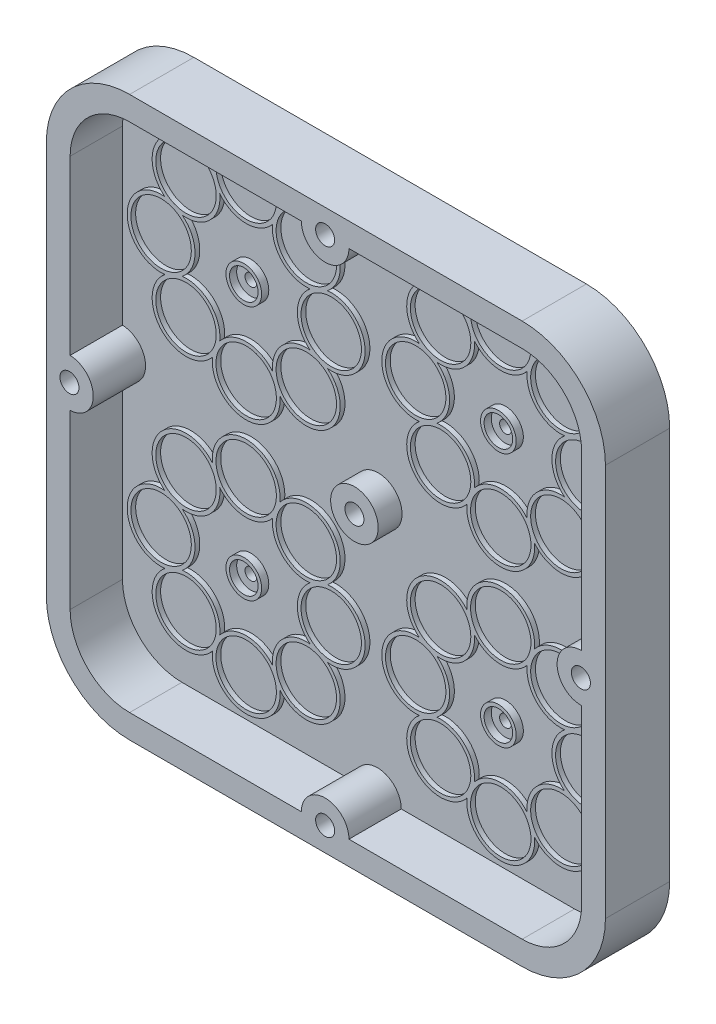
SolidWorks part; units mm, degrees
ref_plane "Front Plane" through (0, 0, 0) normal (0, 0, 1) x (1, 0, 0)
ref_plane "Top Plane" through (0, 0, 0) normal (0, 1, 0) x (1, 0, 0)
ref_plane "Right Plane" through (0, 0, 0) normal (1, 0, 0) x (0, 0, -1)
other "Configuration Table"
sketch "Sketch1" plane through (0, 0, 0) normal (0, 0, 1) x (1, 0, 0)
  line L0 (117.5, 235) -> (117.5, 0) construction
  line L1 (35, 0) -> (200, 0)
  line L2 (0, 35) -> (0, 200)
  line L3 (35, 235) -> (200, 235)
  line L4 (235, 35) -> (235, 200)
  line L5 (0, 117.5) -> (235, 117.5) construction
  line L7 (64, 64) -> (171, 64) construction
  line L8 (64, 64) -> (64, 171) construction
  line L9 (64, 171) -> (171, 171) construction
  line L10 (171, 64) -> (171, 171) construction
  line L11 (64, 64) -> (171, 171) construction
  line L12 (64, 171) -> (171, 64) construction
  arc A0 (200, 0) -> (235, 35) centre (200, 35) ccw
  arc A1 (200, 235) -> (235, 200) centre (200, 200) cw
  arc A2 (35, 0) -> (0, 35) centre (35, 35) cw
  arc A3 (0, 200) -> (35, 235) centre (35, 200) cw
  circle A4 centre (117.5, 225) radius 4
  circle A5 centre (117.5, 10) radius 4
  circle A6 centre (117.5, 117.5) radius 4
  circle A7 centre (225, 117.5) radius 4
  circle A8 centre (10, 117.5) radius 4
  circle A9 centre (64, 171) radius 2.5
  circle A10 centre (171, 171) radius 2.5
  circle A11 centre (171, 64) radius 2.5
  circle A12 centre (64, 64) radius 2.5
  point P7 (235, 0)
  point P12 (0, 0)
  point P15 (0, 235)
  dimension "D3" = 35
  dimension "D4" = 8
  dimension "D5" = 10
  dimension "D6" = 10
  dimension "D7" = 10
  dimension "D8" = 10
  dimension "D11" = 5
  dimension "D1" = 235
  dimension "D2" = 235
  dimension "D9" = 107
  dimension "D10" = 107
extrude "Boss-Extrude1" add sketch "Sketch1" along normal blind 5
sketch "Sketch2" plane through (0, 0, 5) normal (0, 0, 1) x (1, 0, 0)
  line L0 (200, 225) -> (127.186, 225)
  line L1 (10, 200) -> (10, 127.5027)
  line L2 (35, 10) -> (107.186, 10)
  line L3 (225, 35) -> (225, 107.5123)
  line L4 (235, 35) -> (235, 200)
  line L5 (200, 235) -> (35, 235)
  line L6 (0, 200) -> (0, 35)
  line L7 (35, 0) -> (200, 0)
  line L8 (235, 35) -> (235, 200)
  line L9 (200, 235) -> (35, 235)
  line L10 (0, 200) -> (0, 35)
  line L11 (35, 0) -> (200, 0)
  line L12 (10, 107.5104) -> (10, 35)
  line L13 (10, 200) -> (10, 35) construction
  line L14 (107.186, 225) -> (35, 225)
  line L15 (200, 225) -> (35, 225) construction
  line L16 (225, 127.5024) -> (225, 200)
  line L17 (225, 35) -> (225, 200) construction
  line L18 (127.186, 10) -> (200, 10)
  line L19 (35, 10) -> (200, 10) construction
  arc A0 (225, 200) -> (200, 225) centre (200, 200) ccw
  arc A1 (35, 225) -> (10, 200) centre (35, 200) ccw
  arc A2 (10, 35) -> (35, 10) centre (35, 35) ccw
  arc A3 (200, 10) -> (225, 35) centre (200, 35) ccw
  arc A4 (200, 0) -> (235, 35) centre (200, 35) ccw
  arc A5 (235, 200) -> (200, 235) centre (200, 200) ccw
  arc A6 (35, 235) -> (0, 200) centre (35, 200) ccw
  arc A7 (0, 35) -> (35, 0) centre (35, 35) ccw
  arc A8 (200, 0) -> (235, 35) centre (200, 35) ccw
  arc A9 (235, 200) -> (200, 235) centre (200, 200) ccw
  arc A10 (35, 235) -> (0, 200) centre (35, 200) ccw
  arc A11 (0, 35) -> (35, 0) centre (35, 35) ccw
  arc A12 (107.186, 225) -> (127.186, 225) centre (117.186, 225.0074) ccw
  arc A13 (10, 107.5104) -> (10, 127.5027) centre (9.7224, 117.5065) ccw
  arc A15 (225, 127.5024) -> (225, 107.5123) centre (224.686, 117.5074) ccw
  arc A16 (127.186, 10) -> (107.186, 10) centre (117.186, 10.0074) ccw
  circle A17 centre (117.186, 225.0074) radius 4
  circle A18 centre (224.686, 117.5074) radius 4
  circle A19 centre (117.186, 10.0074) radius 4
  circle A20 centre (9.7224, 117.5065) radius 4
  dimension "D1" = 0
  dimension "D2" = 10
extrude "Boss-Extrude2" add sketch "Sketch2" along normal blind 22
sketch "Sketch3" plane through (0, 0, 5) normal (0, 0, 1) x (1, 0, 0)
  circle A0 centre (117.5, 117.5) radius 10
  circle A1 centre (117.5, 117.5) radius 4
  dimension "D1" = 20
extrude "Boss-Extrude3" add sketch "Sketch3" along normal blind 10
sketch "Sketch4" plane through (0, 0, 5) normal (0, 0, 1) x (1, 0, 0)
  line L0 (171, 171) -> (171, 221) construction
  circle A2 centre (171, 171) radius 50 construction
  arc A3 (159.8861, 197.8312) -> (182.1139, 197.8312) centre (171, 206.75) ccw
  circle A4 centre (171, 206.75) radius 12.7
  arc A5 (144.1688, 182.1139) -> (159.8861, 197.8312) centre (145.7209, 196.2791) ccw
  circle A6 centre (145.7209, 196.2791) radius 12.7
  arc A7 (136.8021, 185.1652) -> (136.8021, 156.8348) centre (135.25, 171) ccw
  circle A8 centre (135.25, 171) radius 12.7
  arc A9 (159.8861, 144.1688) -> (144.1688, 159.8861) centre (145.7209, 145.7209) ccw
  circle A10 centre (145.7209, 145.7209) radius 12.7
  arc A11 (182.1139, 144.1688) -> (159.8861, 144.1688) centre (171, 135.25) ccw
  circle A12 centre (171, 135.25) radius 12.7
  arc A13 (197.8312, 159.8861) -> (182.1139, 144.1688) centre (196.2791, 145.7209) ccw
  circle A14 centre (196.2791, 145.7209) radius 12.7
  arc A15 (197.8312, 182.1139) -> (197.8312, 159.8861) centre (206.75, 171) ccw
  circle A16 centre (206.75, 171) radius 12.7
  arc A17 (182.1139, 197.8312) -> (197.8312, 182.1139) centre (196.2791, 196.2791) ccw
  circle A18 centre (196.2791, 196.2791) radius 12.7
  arc A19 (156.8348, 205.1979) -> (136.8021, 185.1652) centre (145.7209, 196.2791) ccw
  arc A20 (185.1652, 205.1979) -> (156.8348, 205.1979) centre (171, 206.75) ccw
  arc A21 (205.1979, 185.1652) -> (185.1652, 205.1979) centre (196.2791, 196.2791) ccw
  arc A22 (205.1979, 156.8348) -> (205.1979, 185.1652) centre (206.75, 171) ccw
  arc A23 (185.1652, 136.8021) -> (205.1979, 156.8348) centre (196.2791, 145.7209) ccw
  arc A24 (156.8348, 136.8021) -> (185.1652, 136.8021) centre (171, 135.25) ccw
  arc A25 (144.1688, 159.8861) -> (144.1688, 182.1139) centre (135.25, 171) ccw
  arc A26 (136.8021, 156.8348) -> (156.8348, 136.8021) centre (145.7209, 145.7209) ccw
  circle A27 centre (117.5, 117.5) radius 17.1573 construction
  circle A28 centre (171, 99.75) radius 12.7
  arc A29 (185.1652, 98.1979) -> (156.8348, 98.1979) centre (171, 99.75) ccw
  arc A30 (156.8348, 98.1979) -> (136.8021, 78.1652) centre (145.7209, 89.2791) ccw
  arc A31 (144.1688, 75.1139) -> (159.8861, 90.8312) centre (145.7209, 89.2791) ccw
  arc A32 (159.8861, 90.8312) -> (182.1139, 90.8312) centre (171, 99.75) ccw
  circle A33 centre (145.7209, 89.2791) radius 12.7
  circle A34 centre (135.25, 64) radius 12.7
  arc A35 (144.1688, 52.8861) -> (144.1688, 75.1139) centre (135.25, 64) ccw
  arc A36 (136.8021, 78.1652) -> (136.8021, 49.8348) centre (135.25, 64) ccw
  arc A37 (159.8861, 37.1688) -> (144.1688, 52.8861) centre (145.7209, 38.7209) ccw
  circle A38 centre (145.7209, 38.7209) radius 12.7
  arc A39 (136.8021, 49.8348) -> (156.8348, 29.8021) centre (145.7209, 38.7209) ccw
  arc A40 (156.8348, 29.8021) -> (185.1652, 29.8021) centre (171, 28.25) ccw
  circle A41 centre (171, 28.25) radius 12.7
  arc A42 (182.1139, 37.1688) -> (159.8861, 37.1688) centre (171, 28.25) ccw
  arc A43 (185.1652, 29.8021) -> (205.1979, 49.8348) centre (196.2791, 38.7209) ccw
  circle A44 centre (196.2791, 38.7209) radius 12.7
  arc A45 (197.8312, 52.8861) -> (182.1139, 37.1688) centre (196.2791, 38.7209) ccw
  arc A46 (205.1979, 49.8348) -> (205.1979, 78.1652) centre (206.75, 64) ccw
  circle A47 centre (206.75, 64) radius 12.7
  arc A48 (197.8312, 75.1139) -> (197.8312, 52.8861) centre (206.75, 64) ccw
  arc A49 (182.1139, 90.8312) -> (197.8312, 75.1139) centre (196.2791, 89.2791) ccw
  circle A50 centre (196.2791, 89.2791) radius 12.7
  arc A51 (205.1979, 78.1652) -> (185.1652, 98.1979) centre (196.2791, 89.2791) ccw
  circle A52 centre (99.75, 64) radius 12.7
  arc A53 (98.1979, 49.8348) -> (98.1979, 78.1652) centre (99.75, 64) ccw
  arc A54 (98.1979, 78.1652) -> (78.1652, 98.1979) centre (89.2791, 89.2791) ccw
  arc A55 (75.1139, 90.8312) -> (90.8312, 75.1139) centre (89.2791, 89.2791) ccw
  arc A56 (90.8312, 75.1139) -> (90.8312, 52.8861) centre (99.75, 64) ccw
  circle A57 centre (89.2791, 89.2791) radius 12.7
  circle A58 centre (64, 99.75) radius 12.7
  arc A59 (52.8861, 90.8312) -> (75.1139, 90.8312) centre (64, 99.75) ccw
  arc A60 (78.1652, 98.1979) -> (49.8348, 98.1979) centre (64, 99.75) ccw
  arc A61 (37.1688, 75.1139) -> (52.8861, 90.8312) centre (38.7209, 89.2791) ccw
  circle A62 centre (38.7209, 89.2791) radius 12.7
  arc A63 (49.8348, 98.1979) -> (29.8021, 78.1652) centre (38.7209, 89.2791) ccw
  arc A64 (29.8021, 78.1652) -> (29.8021, 49.8348) centre (28.25, 64) ccw
  circle A65 centre (28.25, 64) radius 12.7
  arc A66 (37.1688, 52.8861) -> (37.1688, 75.1139) centre (28.25, 64) ccw
  arc A67 (29.8021, 49.8348) -> (49.8348, 29.8021) centre (38.7209, 38.7209) ccw
  circle A68 centre (38.7209, 38.7209) radius 12.7
  arc A69 (52.8861, 37.1688) -> (37.1688, 52.8861) centre (38.7209, 38.7209) ccw
  arc A70 (49.8348, 29.8021) -> (78.1652, 29.8021) centre (64, 28.25) ccw
  circle A71 centre (64, 28.25) radius 12.7
  arc A72 (75.1139, 37.1688) -> (52.8861, 37.1688) centre (64, 28.25) ccw
  arc A73 (90.8312, 52.8861) -> (75.1139, 37.1688) centre (89.2791, 38.7209) ccw
  circle A74 centre (89.2791, 38.7209) radius 12.7
  arc A75 (78.1652, 29.8021) -> (98.1979, 49.8348) centre (89.2791, 38.7209) ccw
  circle A76 centre (64, 135.25) radius 12.7
  arc A77 (49.8348, 136.8021) -> (78.1652, 136.8021) centre (64, 135.25) ccw
  arc A78 (78.1652, 136.8021) -> (98.1979, 156.8348) centre (89.2791, 145.7209) ccw
  arc A79 (90.8312, 159.8861) -> (75.1139, 144.1688) centre (89.2791, 145.7209) ccw
  arc A80 (75.1139, 144.1688) -> (52.8861, 144.1688) centre (64, 135.25) ccw
  circle A81 centre (89.2791, 145.7209) radius 12.7
  circle A82 centre (99.75, 171) radius 12.7
  arc A83 (90.8312, 182.1139) -> (90.8312, 159.8861) centre (99.75, 171) ccw
  arc A84 (98.1979, 156.8348) -> (98.1979, 185.1652) centre (99.75, 171) ccw
  arc A85 (75.1139, 197.8312) -> (90.8312, 182.1139) centre (89.2791, 196.2791) ccw
  circle A86 centre (89.2791, 196.2791) radius 12.7
  arc A87 (98.1979, 185.1652) -> (78.1652, 205.1979) centre (89.2791, 196.2791) ccw
  arc A88 (78.1652, 205.1979) -> (49.8348, 205.1979) centre (64, 206.75) ccw
  circle A89 centre (64, 206.75) radius 12.7
  arc A90 (52.8861, 197.8312) -> (75.1139, 197.8312) centre (64, 206.75) ccw
  arc A91 (49.8348, 205.1979) -> (29.8021, 185.1652) centre (38.7209, 196.2791) ccw
  circle A92 centre (38.7209, 196.2791) radius 12.7
  arc A93 (37.1688, 182.1139) -> (52.8861, 197.8312) centre (38.7209, 196.2791) ccw
  arc A94 (29.8021, 185.1652) -> (29.8021, 156.8348) centre (28.25, 171) ccw
  circle A95 centre (28.25, 171) radius 12.7
  arc A96 (37.1688, 159.8861) -> (37.1688, 182.1139) centre (28.25, 171) ccw
  arc A97 (52.8861, 144.1688) -> (37.1688, 159.8861) centre (38.7209, 145.7209) ccw
  circle A98 centre (38.7209, 145.7209) radius 12.7
  arc A99 (29.8021, 156.8348) -> (49.8348, 136.8021) centre (38.7209, 145.7209) ccw
  dimension "D1" = 4
  dimension "D3" = 100
  dimension "D4" = 28.5
  dimension "D5" = 25.4
  dimension "D6" = 8
extrude "Boss-Extrude4" add sketch "Sketch4" along normal blind 2
sketch "Sketch5" plane through (0, 0, 5) normal (0, 0, 1) x (1, 0, 0)
  circle A0 centre (171, 171) radius 6
  circle A1 centre (171, 171) radius 7.5
  circle A2 centre (64, 171) radius 7.5
  circle A3 centre (64, 171) radius 6
  circle A4 centre (64, 64) radius 7.5
  circle A5 centre (64, 64) radius 6
  circle A6 centre (171, 64) radius 7.5
  circle A7 centre (171, 64) radius 6
  dimension "D1" = 12
  dimension "D2" = 15
extrude "Boss-Extrude5" add sketch "Sketch5" along normal blind 3
